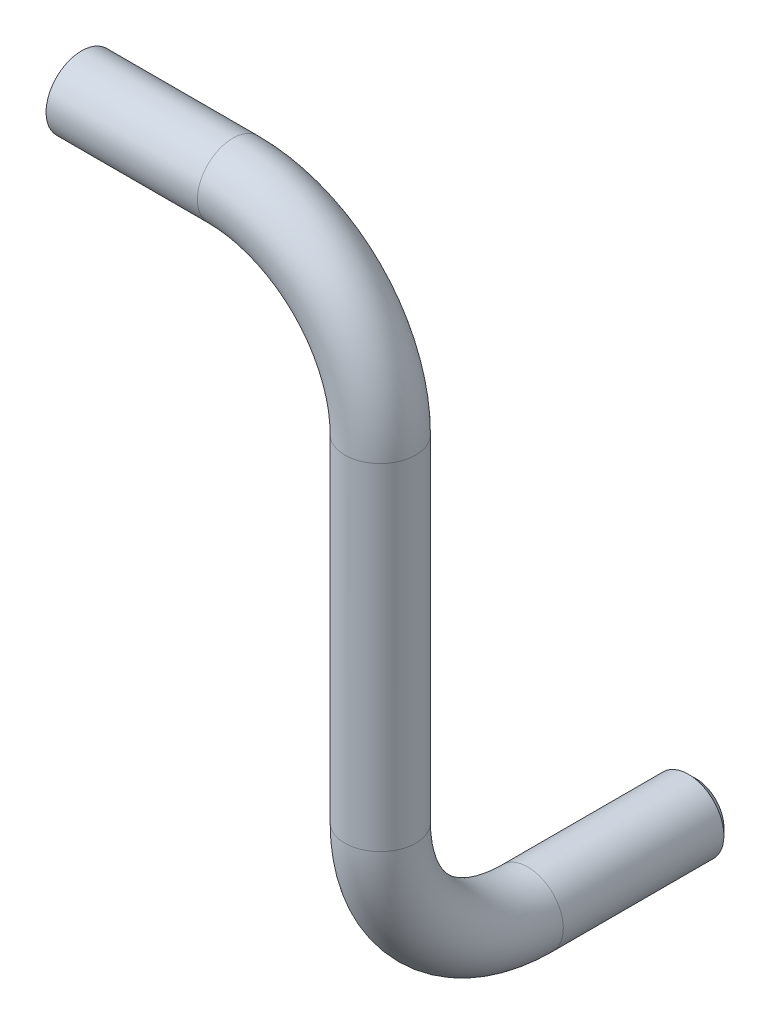
SolidWorks part; units mm, degrees
material "SS400B"
ref_plane "Front Plane" through (0, 0, 0) normal (0, 0, 1) x (1, 0, 0)
ref_plane "Top Plane" through (0, 0, 0) normal (0, 1, 0) x (1, 0, 0)
ref_plane "Right Plane" through (0, 0, 0) normal (1, 0, 0) x (0, 0, -1)
sketch3d "3DSketch1"
  line L0 (0, 0, 0) -> (40.5, 0, 0)
  line L1 (80, -39.5, 0) -> (80, -129.5, 0)
  line L2 (80, -169, -39.5) -> (80, -169, -84.5)
  arc A0 (80, -129.5, 0) -> (80, -169, -39.5) centre (80, -129.5, -39.5) ccw
  arc A1 (40.5, 0, 0) -> (80, -39.5, 0) centre (40.5, -39.5, 0) ccw
  point P7 (80, -169, 0)
  point P8 (119.5, -129.5, -39.5)
  point P11 (80, 0, 0)
  point P12 (40.5, -39.5, -39.5)
  dimension "D4" = 39.5
  dimension "D1" = 80
  dimension "D2" = 169
  dimension "D3" = 84.5
sweep "Sweep1" add path "3DSketch1" circular profile diameter 19 parameters "D3"=19
chamfer "Chamfer1" distance 2 angle 45 1 edges at (89.5, -169, -84.5)
